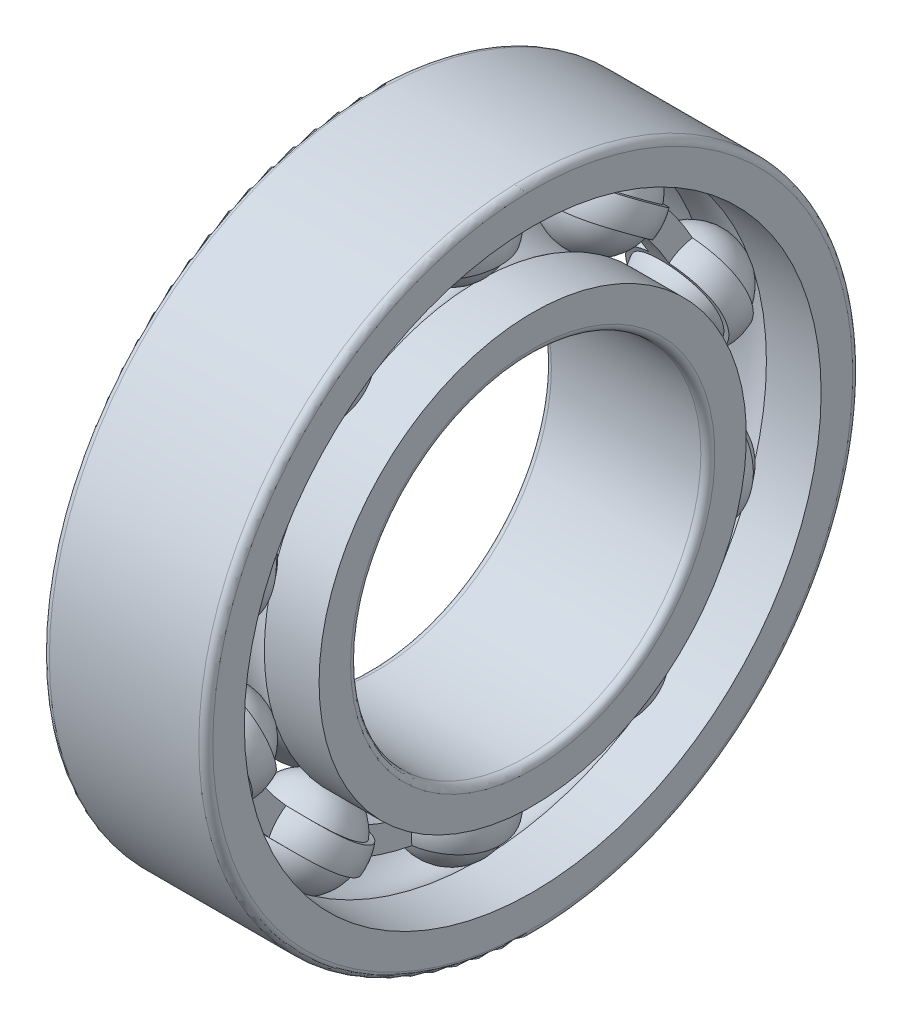
SolidWorks part; units mm, degrees
revolve "凸台-旋转2" add sketch "草图6" angle 360 about L4
sketch "草图6" plane through (0, 0, 0) normal (0, 0, 1) x (1, 0, 0)
  line L0 (0, 0) -> (5.5439, 0) construction
  line L1 (-12.4206, 0) -> (9.8128, 0) construction
  line L2 (0, 0) -> (0, 11.4011) construction
  line L3 (-5.5681, 10.75) -> (6.1049, 10.75) construction
  line L4 (-5.5681, 10.75) -> (6.1049, 10.75) construction
  line L5 (-1.9845, 10.75) -> (1.9845, 10.75)
  arc A0 (-1.9845, 10.75) -> (1.9845, 10.75) centre (0, 10.75) ccw
  dimension "Dw" = 3.969
revolve "基体-旋转" add sketch "草图2" angle 360 about L0
sketch "草图2" plane through (0, 0, 0) normal (0, 0, 1) x (1, 0, 0)
  line L0 (-12.4206, 0) -> (9.8128, 0) construction
  line L1 (0, 0) -> (0, 37.3563) construction
  line L2 (-5.5681, 10.75) -> (6.1049, 10.75) construction
  line L3 (-0.4366, 11.2957) -> (0.4366, 11.2957)
  line L4 (-0.4366, 11.2957) -> (-0.4366, 10.2043)
  line L5 (-0.4366, 10.2043) -> (0.4366, 10.2043)
  line L6 (0.4366, 11.2957) -> (0.4366, 10.2043)
  dimension "D1" = 0.8732
  dimension "D2" = 0.4366
  dimension "D3" = 1.0915
  dimension "D4" = 0.5457
  dimension "D5" = 10.75
revolve "凸台-旋转1" add sketch "草图3" angle 360 about L1
sketch "草图3" plane through (0, 0, 0) normal (0, 0, 1) x (1, 0, 0)
  line L0 (-5.5681, 10.75) -> (6.1049, 10.75) construction
  line L1 (-5.5681, 10.75) -> (6.1049, 10.75) construction
  line L2 (-12.4206, 0) -> (9.8128, 0) construction
  line L3 (-12.4206, 0) -> (9.8128, 0) construction
  line L4 (0, 0) -> (0, 37.3563) construction
  line L5 (0, 0) -> (0, 37.3563) construction
  line L6 (-2.1829, 10.75) -> (2.1829, 10.75)
  arc A0 (-2.1829, 10.75) -> (2.1829, 10.75) centre (0, 10.75) ccw
  dimension "Dwww" = 4.3659
  dimension "D2" = 2.1829
pattern_circular "阵列(圆周)1" count 10 over 360 about axis through (0, 0, 0) along (1, 0, 0) of "凸台-旋转1"
ref_plane "基准面1" through (0, 0, 0) normal (0, 0, 1) x (1, 0, 0)
ref_plane "基准面2" through (0, 0, 0) normal (0, 1, 0) x (1, 0, 0)
ref_plane "基准面3" through (0, 0, 0) normal (1, 0, 0) x (0, 0, -1)
sketch "尺寸草图" plane through (0, 0, 0) normal (0, 0, 1) x (1, 0, 0)
  point P0 (-67.8257, -75.4307)
  point P1 (-63.8567, -75.4307)
  point P2 (-71.0249, 50.7088)
  point P3 (-56.0249, 50.7088)
  point P4 (-43.0249, 50.7088)
  point P5 (-64.0249, 50.7088)
  point P6 (-71.0249, -10.9899)
  point P7 (-52.7249, -10.9899)
  point P8 (-46.3249, -10.9899)
  point P9 (-70.7249, -10.9899)
  point P10 (-57.8257, -75.4307)
sketch "草图4" plane through (0, 0, 0) normal (0, 0, 1) x (1, 0, 0)
  line L0 (0, 0) -> (8.1272, 0) construction
  line L1 (-12.4206, 0) -> (9.8128, 0) construction
  line L3 (-0.4366, 11.2957) -> (0.4366, 11.2957) construction
  line L4 (-2.183, 13.4787) -> (2.1829, 13.4787)
  line L5 (-2.183, 13.4787) -> (-2.183, 11.2957)
  line L6 (-2.183, 11.2957) -> (2.1829, 11.2957)
  line L7 (2.1829, 13.4787) -> (2.1829, 11.2957)
revolve "切除-旋转1" cut sketch "草图4" angle 360 about L0
sketch "草图5" plane through (0, 0, 0) normal (0, 0, 1) x (1, 0, 0)
  line L0 (0, 0) -> (8.2665, 0) construction
  line L1 (-12.4206, 0) -> (9.8128, 0) construction
  line L2 (-0.4366, 10.2043) -> (0.4366, 10.2043) construction
  line L3 (-2.183, 10.2043) -> (2.1829, 10.2043)
  line L4 (-2.183, 10.2043) -> (-2.1829, 8.0213)
  line L5 (-2.1829, 8.0213) -> (2.1829, 8.0213)
  line L6 (2.1829, 10.2043) -> (2.1829, 8.0213)
revolve "切除-旋转2" cut sketch "草图5" angle 360 about L0
pattern_circular "阵列(圆周)2" count 10 over 360 about axis through (0, 0, 0) along (1, 0, 0) of "凸台-旋转2"
sketch "草图7" plane through (0, 0, 0) normal (0, 0, 1) x (1, 0, 0)
  line L0 (0, 0) -> (6.6488, 0) construction
  line L1 (0, 0) -> (0, 16.8954) construction
  line L2 (-3.2, 14) -> (3.2, 14)
  line L3 (-3.5, 13.7) -> (-3.5, 12.35)
  line L4 (-3.5, 12.35) -> (-1.157, 12.35)
  line L5 (3.5, 13.7) -> (3.5, 12.35)
  line L6 (1.157, 12.35) -> (3.5, 12.35)
  arc A0 (-3.2, 14) -> (-3.5, 13.7) centre (-3.2, 13.7) ccw
  arc A1 (3.2, 14) -> (3.5, 13.7) centre (3.2, 13.7) cw
  arc A2 (1.908, 11.2957) -> (-1.908, 11.2957) centre (0, 10.75) ccw construction
  arc A3 (1.174, 12.35) -> (-0.0076, 8.7655) centre (0, 10.75) ccw construction
  arc A4 (1.157, 12.35) -> (-1.157, 12.35) centre (0, 10.75) ccw
  point P10 (-3.5, 14)
  point P13 (3.5, 14)
revolve "凸台-旋转3" add sketch "草图7" angle 360 about L0
sketch "草图8" plane through (0, 0, 0) normal (0, 0, 1) x (1, 0, 0)
  line L0 (-12.4206, 0) -> (9.8128, 0) construction
  line L1 (-12.4206, 0) -> (9.8128, 0) construction
  line L2 (3.5, 13.7) -> (3.5, 12.35) construction
  line L3 (-3.5, 9.15) -> (-1.157, 9.15)
  line L4 (-3.5, 9.15) -> (-3.5, 7.8)
  line L5 (-3.2, 7.5) -> (3.2, 7.5)
  line L6 (3.5, 9.15) -> (3.5, 7.8)
  line L7 (-3.5, 13.7) -> (-3.5, 12.35) construction
  line L8 (1.157, 9.15) -> (3.5, 9.15)
  arc A0 (-3.5, 7.8) -> (-3.2, 7.5) centre (-3.2, 7.8) ccw
  arc A1 (3.2, 7.5) -> (3.5, 7.8) centre (3.2, 7.8) ccw
  arc A2 (-1.908, 10.2043) -> (1.908, 10.2043) centre (0, 10.75) ccw construction
  arc A3 (-1.908, 10.2043) -> (1.908, 10.2043) centre (0, 10.75) ccw construction
  arc A4 (-1.157, 9.15) -> (1.157, 9.15) centre (0, 10.75) ccw
revolve "凸台-旋转4" add sketch "草图8" angle 360 about L1
equation "\"DD@草图8\"=\"d@尺寸草图\""
equation "\"D@草图7\"=\"DD@尺寸草图\""
equation "\"B@草图7\"=\"B@尺寸草图\" "
equation "\"DD2@草图8\"=\"内圈外径DD2@尺寸草图\""
equation "\"D2@草图7\"=\"外圈内径D2@尺寸草图\""
equation "\"R@草图7\"=\"R@尺寸草图\""
equation "\"Dw@草图6\"=\"球径DW@尺寸草图\""
equation "\"Z@阵列(圆周)1\"=\"球数Z@尺寸草图\" "
equation "\"Dwww@草图3\" = 1.1*\"Dw@草图6\""
equation "\"D3@草图2\" = 0.25*\"Dwww@草图3\""
equation "\"D4@草图2\" = \"D3@草图2\"/2"
equation "\"D2@草图3\" = 0.5*\"Dwww@草图3\""
equation "\"D1@草图2\" = 0.2*\"Dwww@草图3\""
equation "\"D2@草图2\" = 0.5*\"D1@草图2\""
equation "\"切除位置@草图4\" = \"Dwww@草图3\"/2"
equation "\"D1@阵列(圆周)2\" = \"Z@阵列(圆周)1\""
equation "\"D3@草图7\" = \"B@草图7\" / 2"
equation "\"D1@草图8\" = \"R@草图7\""
equation "\"D5@草图2\" = 0.25* ( \"D2@草图7\" + \"DD2@草图8\" )  "
